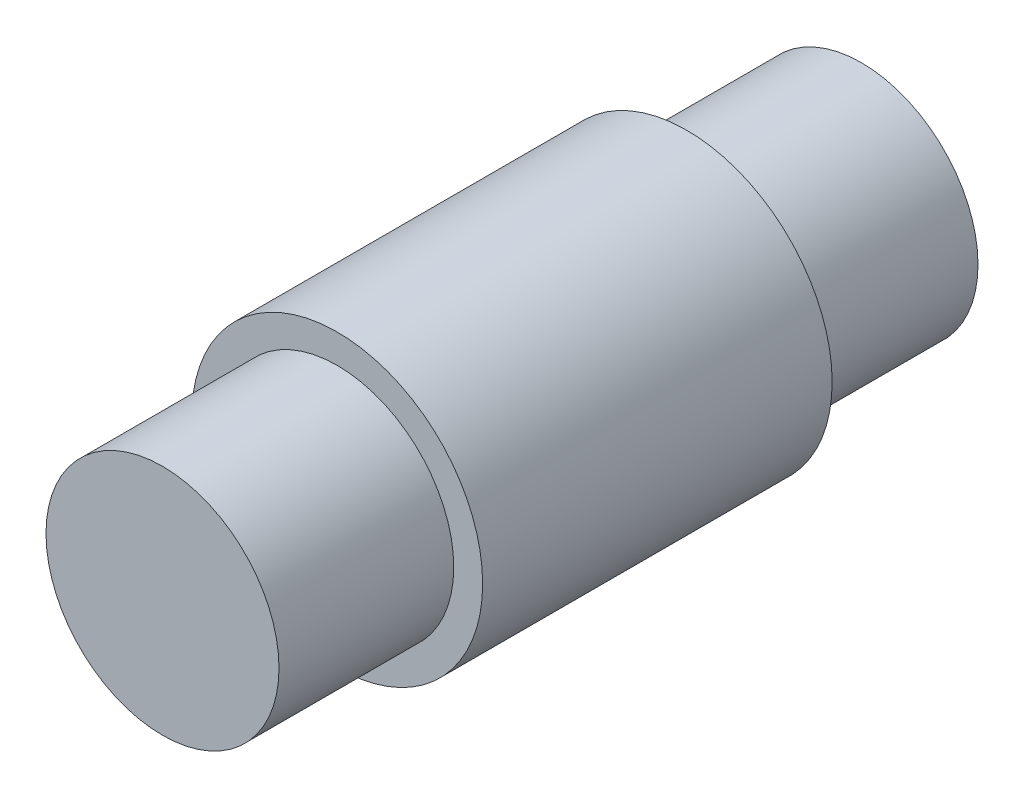
from build123d import *

# Parameters (mm, degrees)
BOSS_EXTRUDE1_DEPTH      = 4.7625
BOSS_EXTRUDE1_DEPTH_BACK = 4.7625
SKETCH1_R                = 3.9624
BOSS_EXTRUDE2_DEPTH      = 9.525
BOSS_EXTRUDE2_DEPTH_BACK = 9.525
BOSS_EXTRUDE2_START      = -4.7625
SKETCH2_R                = 3.175


with BuildPart() as part:
    # Sketch1 → Boss-Extrude1 (new, two sides: drawn at the far end of the back side and taken through both)
    with BuildSketch(Plane.XY.offset(-BOSS_EXTRUDE1_DEPTH_BACK)):
        Circle(SKETCH1_R)
    extrude(amount=BOSS_EXTRUDE1_DEPTH + BOSS_EXTRUDE1_DEPTH_BACK)

    # Sketch2 → Boss-Extrude2 (add, two sides: drawn at the far end of the back side and taken through both)
    with BuildSketch(Plane.XY.offset(4.7625).offset(BOSS_EXTRUDE2_START - BOSS_EXTRUDE2_DEPTH_BACK)):
        Circle(SKETCH2_R)
    extrude(amount=BOSS_EXTRUDE2_DEPTH + BOSS_EXTRUDE2_DEPTH_BACK)


solid = part.part
